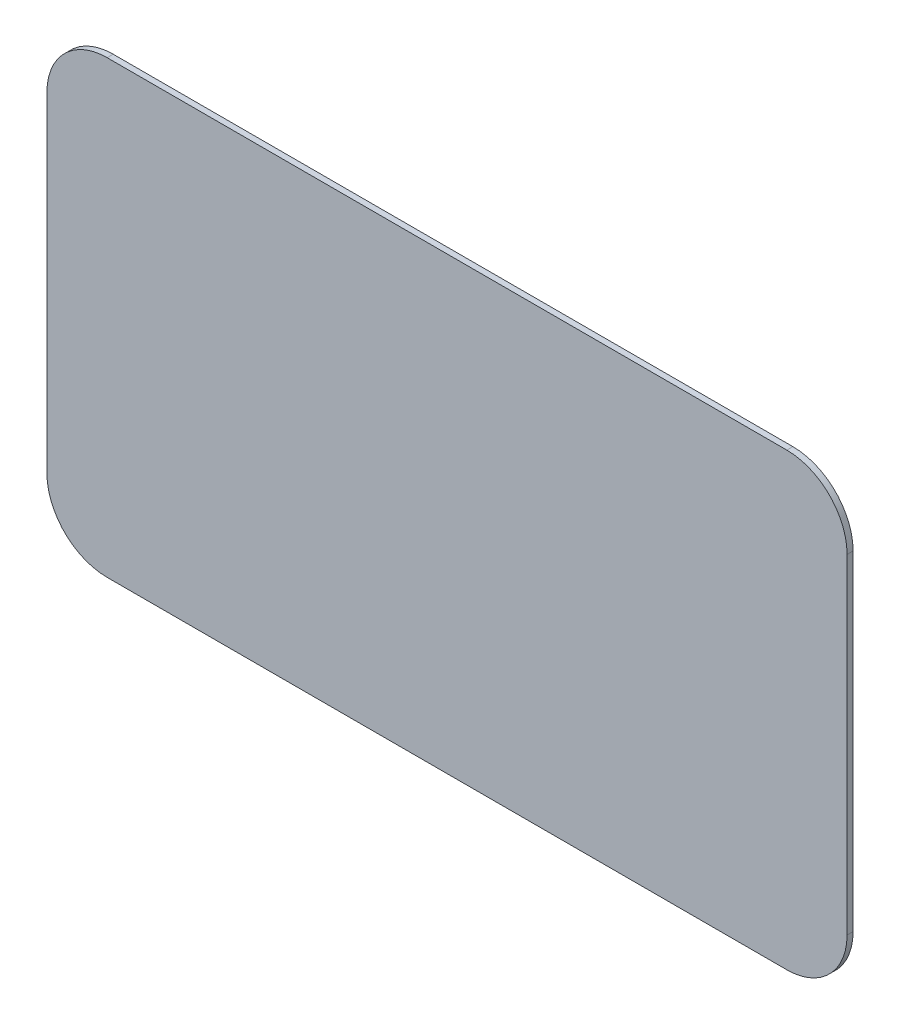
SolidWorks part; units mm, degrees
ref_plane "Front Plane" through (0, 0, 0) normal (0, 0, 1) x (1, 0, 0)
ref_plane "Top Plane" through (0, 0, 0) normal (0, 1, 0) x (1, 0, 0)
ref_plane "Right Plane" through (0, 0, 0) normal (1, 0, 0) x (0, 0, -1)
sketch "Sketch1" plane through (0, 0, 0) normal (0, 0, 1) x (1, 0, 0)
  line L1 (-66.4, -37.35) -> (66.4, -37.35)
  line L2 (-66.4, -37.35) -> (-66.4, 37.35)
  line L3 (-66.4, 37.35) -> (66.4, 37.35)
  line L4 (66.4, -37.35) -> (66.4, 37.35)
  line L5 (-66.4, -37.35) -> (66.4, 37.35) construction
  line L6 (-66.4, 37.35) -> (66.4, -37.35) construction
  point P0 (0, 0)
  dimension "D1" = 132.8
  dimension "D2" = 74.7
extrude "Boss-Extrude1" add sketch "Sketch1" along normal blind 1 contours L3 L4 L1 L2
fillet "Fillet1" radius 10 4 edges at (66.4, 37.35, 0.5) (66.4, -37.35, 0.5) (-66.4, 37.35, 0.5) (-66.4, -37.35, 0.5)
